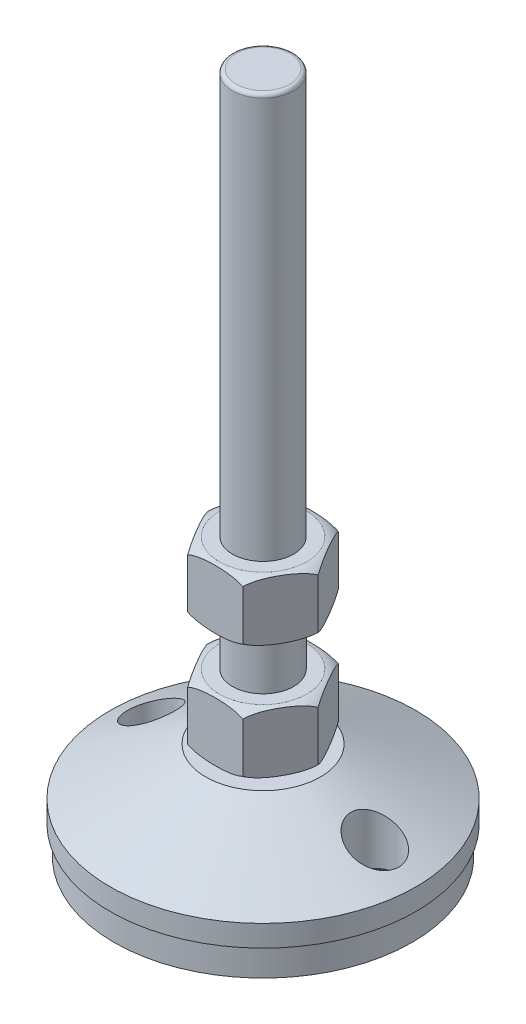
from build123d import *

# Parameters (mm, degrees)
HOLE_WIZARD_12_0_12_1_D            = 12
EXTRUDE_1_DEPTH                    = 16
PATTERN_LINEAR_1_COUNT             = 2
PATTERN_LINEAR_1_PITCH             = 30
SKETCH_9_W                         = 6.25
SKETCH_9_H                         = 171
HOLE_WIZARD_12_5_12_5_1_AT_2_COUNT = 2
HOLE_WIZARD_12_5_12_5_1_AT_2_PITCH = 58.5
FILLET_1_R                         = 1


with BuildPart() as part:
    # 草图1 → 旋转1 (revolve)
    with BuildSketch(Plane.XY, mode=Mode.PRIVATE) as revolve_1_sk:
        Polygon((18.76070467, 7.5), (13.396780619, 18.8), (8, 18.8), (8, 15.8), (11.5, 15.8), (19, 0), (39, 0), (39, 7.5), align=None)
    revolve(revolve_1_sk.sketch.rotate(Axis((0, -6.214285714, 0), (0, 1, 0)), 90), axis=Axis((0, -6.214285714, 0), (0, 1, 0)))

    # Ø12.0 (12) 直径孔1 (through all)
    with Locations(Plane(origin=(0, 7.5, 0), x_dir=(1, 0, 0), z_dir=(0, 1, 0))):
        with Locations((-29.25, 0), (29.25, 0)):
            Hole(HOLE_WIZARD_12_0_12_1_D / 2)


with BuildPart() as body_2:
    # 草图2 → 旋转2 (revolve)
    with BuildSketch(Plane.XY, mode=Mode.PRIVATE) as revolve_2_sk:
        Polygon((-40, 7.5), (-18.76070467, 7.5), (-13.396780619, 18.8), (-8, 18.8), (-8, 15.8), (-11, 15.8), (-11, 8.3), (0, 8.3), (0, 178.5), (-8, 178.5), (-8, 25.5), (-15, 25.5), (-40, 13.1), align=None)
    revolve(revolve_2_sk.sketch.rotate(Axis((0, -3.872490415, 0), (0, 1, 0)), 270), axis=Axis((0, -3.872490415, 0), (0, 1, 0)))

    # 草图6 → 凸台-拉伸1 (add)
    with BuildSketch(Plane(origin=(0, 26.5, 0), x_dir=(1, 0, 0), z_dir=(0, 1, 0))):
        Polygon((14.43375673, 0), (7.216878365, 12.5), (-7.216878365, 12.5), (-14.43375673, 0), (-7.216878365, -12.5), (7.216878365, -12.5), align=None)
    extrude_1 = extrude(amount=EXTRUDE_1_DEPTH)

    # 草图7 → 切除-旋转1 (revolve, cut)
    with BuildSketch(Plane.XY, mode=Mode.PRIVATE) as cut_revolve_1_sk:
        with BuildLine():
            Line((14.43375673, 42.5), (11.43375673, 42.5))
            ThreePointArc((11.43375673, 42.5), (13.040703697, 41.963893935), (14.43375673, 41))
            Line((14.43375673, 41), (14.43375673, 42.5))
        make_face()
        with BuildLine():
            Line((14.43375673, 26.5), (14.43375673, 28))
            ThreePointArc((14.43375673, 28), (13.040703697, 27.036106065), (11.43375673, 26.5))
            Line((11.43375673, 26.5), (14.43375673, 26.5))
        make_face()
    cut_revolve_1 = revolve(cut_revolve_1_sk.sketch.rotate(Axis((0, -6.467317027, 0), (0, 1, 0)), 90), axis=Axis((0, -6.467317027, 0), (0, 1, 0)), mode=Mode.SUBTRACT)

    # 阵列(线性)1: 凸台-拉伸1, 切除-旋转1 ×2
    with Locations(*[(0, i * PATTERN_LINEAR_1_PITCH, 0) for i in range(1, PATTERN_LINEAR_1_COUNT)]):
        add(extrude_1)
        add(cut_revolve_1, mode=Mode.SUBTRACT)

    # 草图9 → Ø12.5 (12.5) 直径孔1 (revolve, cut)
    with BuildSketch(Plane(origin=(29.25, 7.5, 0), x_dir=(0, 0, -1), z_dir=(1, 0, 0))):
        with Locations((3.125, 85.5)):
            Rectangle(SKETCH_9_W, SKETCH_9_H)
    hole_wizard_12_5_12_5_1 = revolve(axis=Axis((29.25, 1.15, 0), (0, 1, 0)), mode=Mode.SUBTRACT)

    # Ø12.5 (12.5) 直径孔1 at 2: Ø12.5 (12.5) 直径孔1 ×2
    with Locations(*[(-i * HOLE_WIZARD_12_5_12_5_1_AT_2_PITCH, 0, 0) for i in range(1, HOLE_WIZARD_12_5_12_5_1_AT_2_COUNT)]):
        add(hole_wizard_12_5_12_5_1, mode=Mode.SUBTRACT)

    # 圆角1
    fillet_1_edges = [body_2.edges().sort_by_distance(p)[0] for p in [
        (0, 178.5, 8),
    ]]
    fillet(fillet_1_edges, radius=FILLET_1_R)


solid = Compound([part.part, body_2.part])
